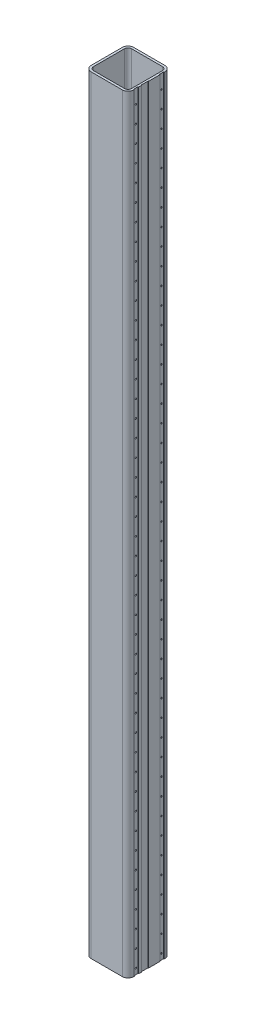
SolidWorks part; units mm, degrees
ref_plane "Front Plane" through (0, 0, 0) normal (0, 0, 1) x (1, 0, 0)
ref_plane "Top Plane" through (0, 0, 0) normal (0, 1, 0) x (1, 0, 0)
ref_plane "Right Plane" through (0, 0, 0) normal (1, 0, 0) x (0, 0, -1)
sketch "Sketch1" plane through (0, 0, 0) normal (0, 1, 0) x (1, 0, 0)
  line L0 (-67, -55) -> (-67, 55)
  line L1 (-55, -75) -> (55, -75)
  line L2 (-75, -55) -> (-75, 55)
  line L3 (-55, 75) -> (55, 75)
  line L4 (75, -55) -> (75, 55)
  line L5 (-75, -75) -> (75, 75) construction
  line L6 (-75, 75) -> (75, -75) construction
  line L7 (-55, 67) -> (55, 67)
  line L8 (67, -55) -> (67, 55)
  line L9 (-55, -67) -> (55, -67)
  arc A0 (55, -75) -> (75, -55) centre (55, -55) ccw
  arc A1 (55, 75) -> (75, 55) centre (55, 55) cw
  arc A2 (-75, 55) -> (-55, 75) centre (-55, 55) cw
  arc A3 (-55, -75) -> (-75, -55) centre (-55, -55) cw
  arc A4 (-67, 55) -> (-55, 67) centre (-55, 55) cw
  arc A5 (55, 67) -> (67, 55) centre (55, 55) cw
  arc A6 (55, -67) -> (67, -55) centre (55, -55) ccw
  arc A7 (-55, -67) -> (-67, -55) centre (-55, -55) cw
  point P0 (0, 0)
  dimension "D3" = 20
  dimension "D1" = 150
  dimension "D2" = 150
  dimension "D4" = 8
extrude "Boss-Extrude1" add sketch "Sketch1" along normal mid plane 2710
sketch "Sketch2" plane through (0, -1355, 0) normal (0, -1, 0) x (1, 0, 0)
  line L0 (75, 55) -> (75, -55) construction
  line L1 (75, 52.7) -> (73, 52.7)
  line L2 (75, 52.7) -> (75, 37.7)
  line L3 (75, 37.7) -> (73, 37.7)
  line L4 (73, 52.7) -> (73, 37.7)
  line L5 (0, 0) -> (75, 0) construction
  line L6 (75, -37.7) -> (73, -37.7)
  line L7 (75, -37.7) -> (75, -52.7)
  line L8 (75, -52.7) -> (73, -52.7)
  line L9 (73, -37.7) -> (73, -52.7)
  line L11 (75, 27.2) -> (73.5, 27.2)
  line L12 (75, 27.2) -> (75, 2.2)
  line L13 (75, 2.2) -> (73.5, 2.2)
  line L14 (73.5, 27.2) -> (73.5, 2.2)
  dimension "D1" = 2
  dimension "D2" = 15
  dimension "D3" = 15
  dimension "D4" = 2
  dimension "D5" = 37.7
  dimension "D6" = 37.7
  dimension "D7" = 1.5
  dimension "D8" = 25
  dimension "D9" = 10.5
extrude "Cut-Extrude1" cut sketch "Sketch2" against normal blind 4000
sketch "Sketch4" plane through (73, 0, 0) normal (1, 0, 0) x (0, 0, -1)
  line L0 (-52.7, -1355) -> (-37.7, -1355) construction
  circle A0 centre (-45.2, -1335) radius 2.6
  dimension "D1" = 5.2
  dimension "D2" = 20
  dimension "D3" = 45.2
extrude "Cut-Extrude2" cut sketch "Sketch4" against normal up to next
pattern_linear "LPattern2" count 2 spacing 90.4 along (0, 0, -1) count 45 spacing 60 along (0, 1, 0) of "Cut-Extrude2"
